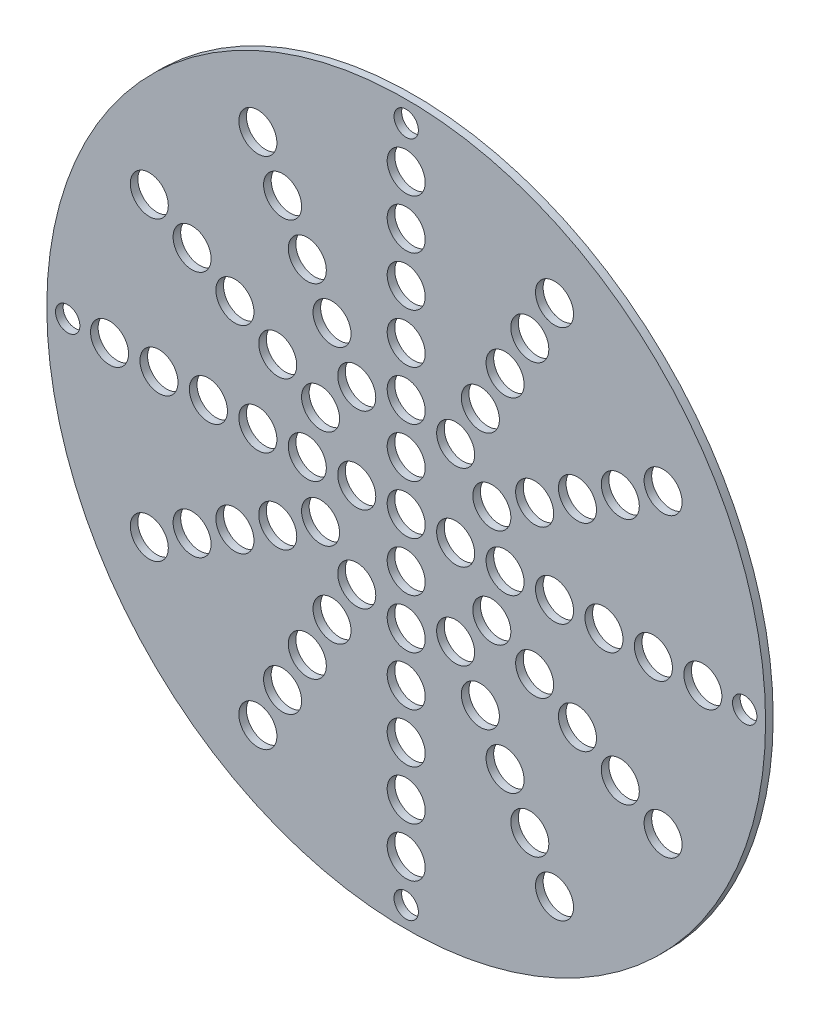
from build123d import *

# Parameters (mm, degrees)
SKETCH_1_R          = 47.25
EXTRUDE_1_DEPTH     = 1
SKETCH_6_R          = 2.5
CUT_EXTRUDE_3_DEPTH = 2
SKETCH_7_R          = 1.6
CUT_EXTRUDE_4_DEPTH = 2


with BuildPart() as part:
    # 草图1 → 凸台-拉伸1 (new body)
    with BuildSketch(Plane.XY):
        Circle(SKETCH_1_R)
    extrude(amount=EXTRUDE_1_DEPTH)

    # 草图6 → 切除-拉伸3 (cut)
    with BuildSketch(Plane.XY.offset(1)):
        with Locations((0, 6.5)):
            Circle(SKETCH_6_R)
        with Locations((0, 13)):
            Circle(SKETCH_6_R)
        with Locations((0, 19.5)):
            Circle(SKETCH_6_R)
        with Locations((0, 26)):
            Circle(SKETCH_6_R)
        with Locations((0, 32.5)):
            Circle(SKETCH_6_R)
        with Locations((0, 39)):
            Circle(SKETCH_6_R)
        Circle(SKETCH_6_R)
        with Locations((19.5, 33.774990748)):
            Circle(SKETCH_6_R)
        with Locations((16.25, 28.145825623)):
            Circle(SKETCH_6_R)
        with Locations((13, 22.516660498)):
            Circle(SKETCH_6_R)
        with Locations((9.75, 16.887495374)):
            Circle(SKETCH_6_R)
        with Locations((6.5, 11.258330249)):
            Circle(SKETCH_6_R)
        with Locations((33.774990748, 19.5)):
            Circle(SKETCH_6_R)
        with Locations((28.145825623, 16.25)):
            Circle(SKETCH_6_R)
        with Locations((22.516660498, 13)):
            Circle(SKETCH_6_R)
        with Locations((16.887495374, 9.75)):
            Circle(SKETCH_6_R)
        with Locations((11.258330249, 6.5)):
            Circle(SKETCH_6_R)
        with Locations((39, 0)):
            Circle(SKETCH_6_R)
        with Locations((32.5, 0)):
            Circle(SKETCH_6_R)
        with Locations((26, 0)):
            Circle(SKETCH_6_R)
        with Locations((19.5, 0)):
            Circle(SKETCH_6_R)
        with Locations((13, 0)):
            Circle(SKETCH_6_R)
        with Locations((33.774990748, -19.5)):
            Circle(SKETCH_6_R)
        with Locations((28.145825623, -16.25)):
            Circle(SKETCH_6_R)
        with Locations((22.516660498, -13)):
            Circle(SKETCH_6_R)
        with Locations((16.887495374, -9.75)):
            Circle(SKETCH_6_R)
        with Locations((11.258330249, -6.5)):
            Circle(SKETCH_6_R)
        with Locations((19.5, -33.774990748)):
            Circle(SKETCH_6_R)
        with Locations((16.25, -28.145825623)):
            Circle(SKETCH_6_R)
        with Locations((13, -22.516660498)):
            Circle(SKETCH_6_R)
        with Locations((9.75, -16.887495374)):
            Circle(SKETCH_6_R)
        with Locations((6.5, -11.258330249)):
            Circle(SKETCH_6_R)
        with Locations((0, -39)):
            Circle(SKETCH_6_R)
        with Locations((0, -32.5)):
            Circle(SKETCH_6_R)
        with Locations((0, -26)):
            Circle(SKETCH_6_R)
        with Locations((0, -19.5)):
            Circle(SKETCH_6_R)
        with Locations((0, -13)):
            Circle(SKETCH_6_R)
        with Locations((-19.5, -33.774990748)):
            Circle(SKETCH_6_R)
        with Locations((-16.25, -28.145825623)):
            Circle(SKETCH_6_R)
        with Locations((-13, -22.516660498)):
            Circle(SKETCH_6_R)
        with Locations((-9.75, -16.887495374)):
            Circle(SKETCH_6_R)
        with Locations((-6.5, -11.258330249)):
            Circle(SKETCH_6_R)
        with Locations((-33.774990748, -19.5)):
            Circle(SKETCH_6_R)
        with Locations((-28.145825623, -16.25)):
            Circle(SKETCH_6_R)
        with Locations((-22.516660498, -13)):
            Circle(SKETCH_6_R)
        with Locations((-16.887495374, -9.75)):
            Circle(SKETCH_6_R)
        with Locations((-11.258330249, -6.5)):
            Circle(SKETCH_6_R)
        with Locations((-39, 0)):
            Circle(SKETCH_6_R)
        with Locations((-32.5, 0)):
            Circle(SKETCH_6_R)
        with Locations((-26, 0)):
            Circle(SKETCH_6_R)
        with Locations((-19.5, 0)):
            Circle(SKETCH_6_R)
        with Locations((-13, 0)):
            Circle(SKETCH_6_R)
        with Locations((-33.774990748, 19.5)):
            Circle(SKETCH_6_R)
        with Locations((-28.145825623, 16.25)):
            Circle(SKETCH_6_R)
        with Locations((-22.516660498, 13)):
            Circle(SKETCH_6_R)
        with Locations((-16.887495374, 9.75)):
            Circle(SKETCH_6_R)
        with Locations((-11.258330249, 6.5)):
            Circle(SKETCH_6_R)
        with Locations((-19.5, 33.774990748)):
            Circle(SKETCH_6_R)
        with Locations((-16.25, 28.145825623)):
            Circle(SKETCH_6_R)
        with Locations((-13, 22.516660498)):
            Circle(SKETCH_6_R)
        with Locations((-9.75, 16.887495374)):
            Circle(SKETCH_6_R)
        with Locations((-6.5, 11.258330249)):
            Circle(SKETCH_6_R)
        with Locations((6.5, 0)):
            Circle(SKETCH_6_R)
        with Locations((0, -6.5)):
            Circle(SKETCH_6_R)
        with Locations((-6.5, 0)):
            Circle(SKETCH_6_R)
    extrude(amount=-CUT_EXTRUDE_3_DEPTH, mode=Mode.SUBTRACT)

    # 草图7 → 切除-拉伸4 (cut)
    with BuildSketch(Plane.XY.offset(1)):
        with Locations((0, -44.5)):
            Circle(SKETCH_7_R)
        with Locations((44.5, 0)):
            Circle(SKETCH_7_R)
        with Locations((-44.5, 0)):
            Circle(SKETCH_7_R)
        with Locations((0, 44.5)):
            Circle(SKETCH_7_R)
    extrude(amount=-CUT_EXTRUDE_4_DEPTH, mode=Mode.SUBTRACT)


solid = part.part
